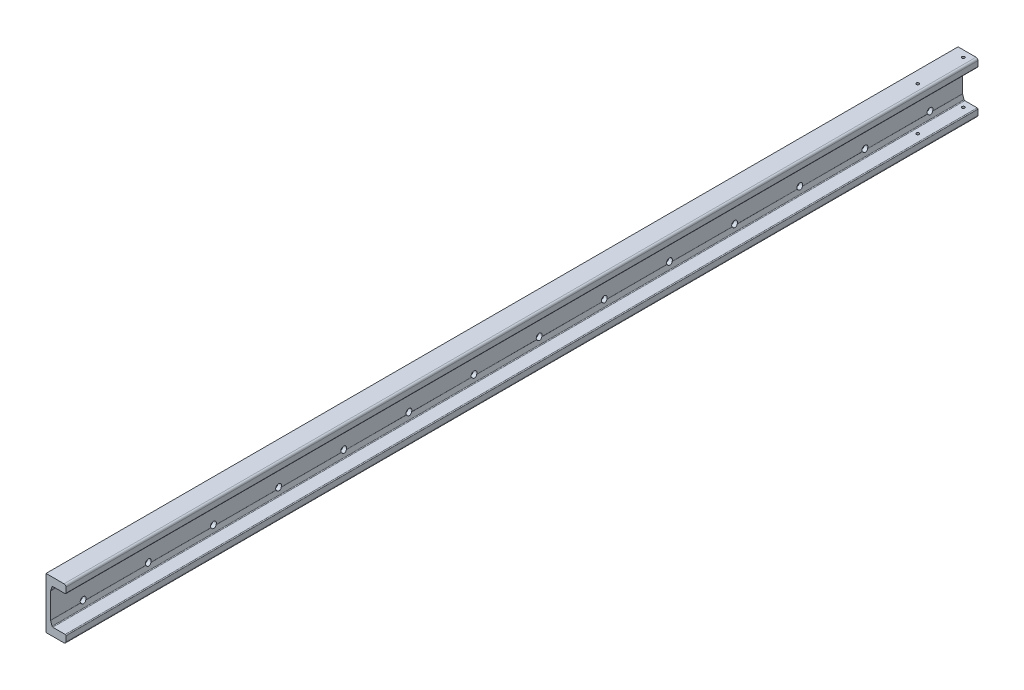
from build123d import *

# Parameters (mm, degrees)
EXTRUDE_1_DEPTH     = 2800
FILLET_1_R          = 6
FILLET_2_R          = 2.5
SKETCH_2_R          = 5.5
CUT_EXTRUDE_1_DEPTH = 3
SKETCH_3_R          = 9
CUT_EXTRUDE_2_DEPTH = 31
HOLE_WIZARD_M10_1_D = 8.5


with BuildPart() as part:
    # 草图1 → 凸台-拉伸1 (new body)
    with BuildSketch(Plane.XY):
        Polygon((0, 0), (-61.2, 0), (-61.2, -157.2), (0, -157.2), (0, -132.8), (-42.2, -132.8), (-47.2, -117.8), (-47.2, -39.4), (-42.2, -24.4), (0, -24.4), align=None)
    extrude(amount=EXTRUDE_1_DEPTH)

    # 圆角1
    fillet_1_edges = [part.edges().sort_by_distance(p)[0] for p in [
        (0, -157.2, 1400),
        (0, 0, 1400),
    ]]
    fillet(fillet_1_edges, radius=FILLET_1_R)

    # 圆角2
    fillet_2_edges = [part.edges().sort_by_distance(p)[0] for p in [
        (-47.2, -39.4, 1400),
        (-47.2, -117.8, 1400),
        (-42.2, -132.8, 1400),
        (0, -132.8, 1400),
        (0, -24.4, 1400),
        (-42.2, -24.4, 1400),
    ]]
    fillet(fillet_2_edges, radius=FILLET_2_R)

    # 草图2 → 切除-拉伸1 (cut)
    with BuildSketch(Plane.ZY.offset(61.2)):
        with Locations(Location((100, -113.6, 0), (0, 0, 270))):
            Circle(SKETCH_2_R)
        with Locations(Location((100, -43.6, 0), (0, 0, 270))):
            Circle(SKETCH_2_R)
        with Locations(Location((300, -43.6, 0), (0, 0, 270))):
            Circle(SKETCH_2_R)
        with Locations(Location((300, -113.6, 0), (0, 0, 270))):
            Circle(SKETCH_2_R)
        with Locations(Location((500, -43.6, 0), (0, 0, 270))):
            Circle(SKETCH_2_R)
        with Locations(Location((500, -113.6, 0), (0, 0, 270))):
            Circle(SKETCH_2_R)
        with Locations(Location((700, -43.6, 0), (0, 0, 270))):
            Circle(SKETCH_2_R)
        with Locations(Location((700, -113.6, 0), (0, 0, 270))):
            Circle(SKETCH_2_R)
        with Locations(Location((900, -43.6, 0), (0, 0, 270))):
            Circle(SKETCH_2_R)
        with Locations(Location((900, -113.6, 0), (0, 0, 270))):
            Circle(SKETCH_2_R)
        with Locations(Location((1100, -43.6, 0), (0, 0, 270))):
            Circle(SKETCH_2_R)
        with Locations(Location((1100, -113.6, 0), (0, 0, 270))):
            Circle(SKETCH_2_R)
        with Locations(Location((1300, -43.6, 0), (0, 0, 270))):
            Circle(SKETCH_2_R)
        with Locations(Location((1300, -113.6, 0), (0, 0, 270))):
            Circle(SKETCH_2_R)
        with Locations(Location((1500, -43.6, 0), (0, 0, 270))):
            Circle(SKETCH_2_R)
        with Locations(Location((1500, -113.6, 0), (0, 0, 270))):
            Circle(SKETCH_2_R)
        with Locations(Location((1700, -43.6, 0), (0, 0, 270))):
            Circle(SKETCH_2_R)
        with Locations(Location((1700, -113.6, 0), (0, 0, 270))):
            Circle(SKETCH_2_R)
        with Locations(Location((1900, -43.6, 0), (0, 0, 270))):
            Circle(SKETCH_2_R)
        with Locations(Location((1900, -113.6, 0), (0, 0, 270))):
            Circle(SKETCH_2_R)
        with Locations(Location((2100, -43.6, 0), (0, 0, 270))):
            Circle(SKETCH_2_R)
        with Locations(Location((2100, -113.6, 0), (0, 0, 270))):
            Circle(SKETCH_2_R)
        with Locations(Location((2300, -43.6, 0), (0, 0, 270))):
            Circle(SKETCH_2_R)
        with Locations(Location((2300, -113.6, 0), (0, 0, 270))):
            Circle(SKETCH_2_R)
        with Locations(Location((2500, -43.6, 0), (0, 0, 270))):
            Circle(SKETCH_2_R)
        with Locations(Location((2500, -113.6, 0), (0, 0, 270))):
            Circle(SKETCH_2_R)
        with Locations(Location((2700, -43.6, 0), (0, 0, 270))):
            Circle(SKETCH_2_R)
        with Locations(Location((2700, -113.6, 0), (0, 0, 270))):
            Circle(SKETCH_2_R)
    extrude(amount=-CUT_EXTRUDE_1_DEPTH, mode=Mode.SUBTRACT)

    # 草图3 → 切除-拉伸2 (cut)
    with BuildSketch(Plane.ZY.offset(58.2)):
        with Locations(Location((100, -43.6, 0), (0, 0, 270))):
            Circle(SKETCH_3_R)
        with Locations(Location((100, -113.6, 0), (0, 0, 270))):
            Circle(SKETCH_3_R)
        with Locations(Location((300, -43.6, 0), (0, 0, 270))):
            Circle(SKETCH_3_R)
        with Locations(Location((300, -113.6, 0), (0, 0, 270))):
            Circle(SKETCH_3_R)
        with Locations(Location((500, -43.6, 0), (0, 0, 270))):
            Circle(SKETCH_3_R)
        with Locations(Location((500, -113.6, 0), (0, 0, 270))):
            Circle(SKETCH_3_R)
        with Locations(Location((700, -43.6, 0), (0, 0, 270))):
            Circle(SKETCH_3_R)
        with Locations(Location((700, -113.6, 0), (0, 0, 270))):
            Circle(SKETCH_3_R)
        with Locations(Location((900, -43.6, 0), (0, 0, 270))):
            Circle(SKETCH_3_R)
        with Locations(Location((900, -113.6, 0), (0, 0, 270))):
            Circle(SKETCH_3_R)
        with Locations(Location((1100, -43.6, 0), (0, 0, 270))):
            Circle(SKETCH_3_R)
        with Locations(Location((1100, -113.6, 0), (0, 0, 270))):
            Circle(SKETCH_3_R)
        with Locations(Location((1300, -43.6, 0), (0, 0, 270))):
            Circle(SKETCH_3_R)
        with Locations(Location((1300, -113.6, 0), (0, 0, 270))):
            Circle(SKETCH_3_R)
        with Locations(Location((1500, -43.6, 0), (0, 0, 270))):
            Circle(SKETCH_3_R)
        with Locations(Location((1500, -113.6, 0), (0, 0, 270))):
            Circle(SKETCH_3_R)
        with Locations(Location((1700, -43.6, 0), (0, 0, 270))):
            Circle(SKETCH_3_R)
        with Locations(Location((1700, -113.6, 0), (0, 0, 270))):
            Circle(SKETCH_3_R)
        with Locations(Location((1900, -43.6, 0), (0, 0, 270))):
            Circle(SKETCH_3_R)
        with Locations(Location((1900, -113.6, 0), (0, 0, 270))):
            Circle(SKETCH_3_R)
        with Locations(Location((2100, -43.6, 0), (0, 0, 270))):
            Circle(SKETCH_3_R)
        with Locations(Location((2100, -113.6, 0), (0, 0, 270))):
            Circle(SKETCH_3_R)
        with Locations(Location((2300, -43.6, 0), (0, 0, 270))):
            Circle(SKETCH_3_R)
        with Locations(Location((2300, -113.6, 0), (0, 0, 270))):
            Circle(SKETCH_3_R)
        with Locations(Location((2500, -43.6, 0), (0, 0, 270))):
            Circle(SKETCH_3_R)
        with Locations(Location((2500, -113.6, 0), (0, 0, 270))):
            Circle(SKETCH_3_R)
        with Locations(Location((2700, -43.6, 0), (0, 0, 270))):
            Circle(SKETCH_3_R)
        with Locations(Location((2700, -113.6, 0), (0, 0, 270))):
            Circle(SKETCH_3_R)
    extrude(amount=-CUT_EXTRUDE_2_DEPTH, mode=Mode.SUBTRACT)

    # M10 螺纹孔1 (through all)
    with Locations(Plane(origin=(0, 0, 0), x_dir=(1, 0, 0), z_dir=(0, 1, 0))):
        with Locations((-25, -20), (-25, -160)):
            Hole(HOLE_WIZARD_M10_1_D / 2)


solid = part.part
